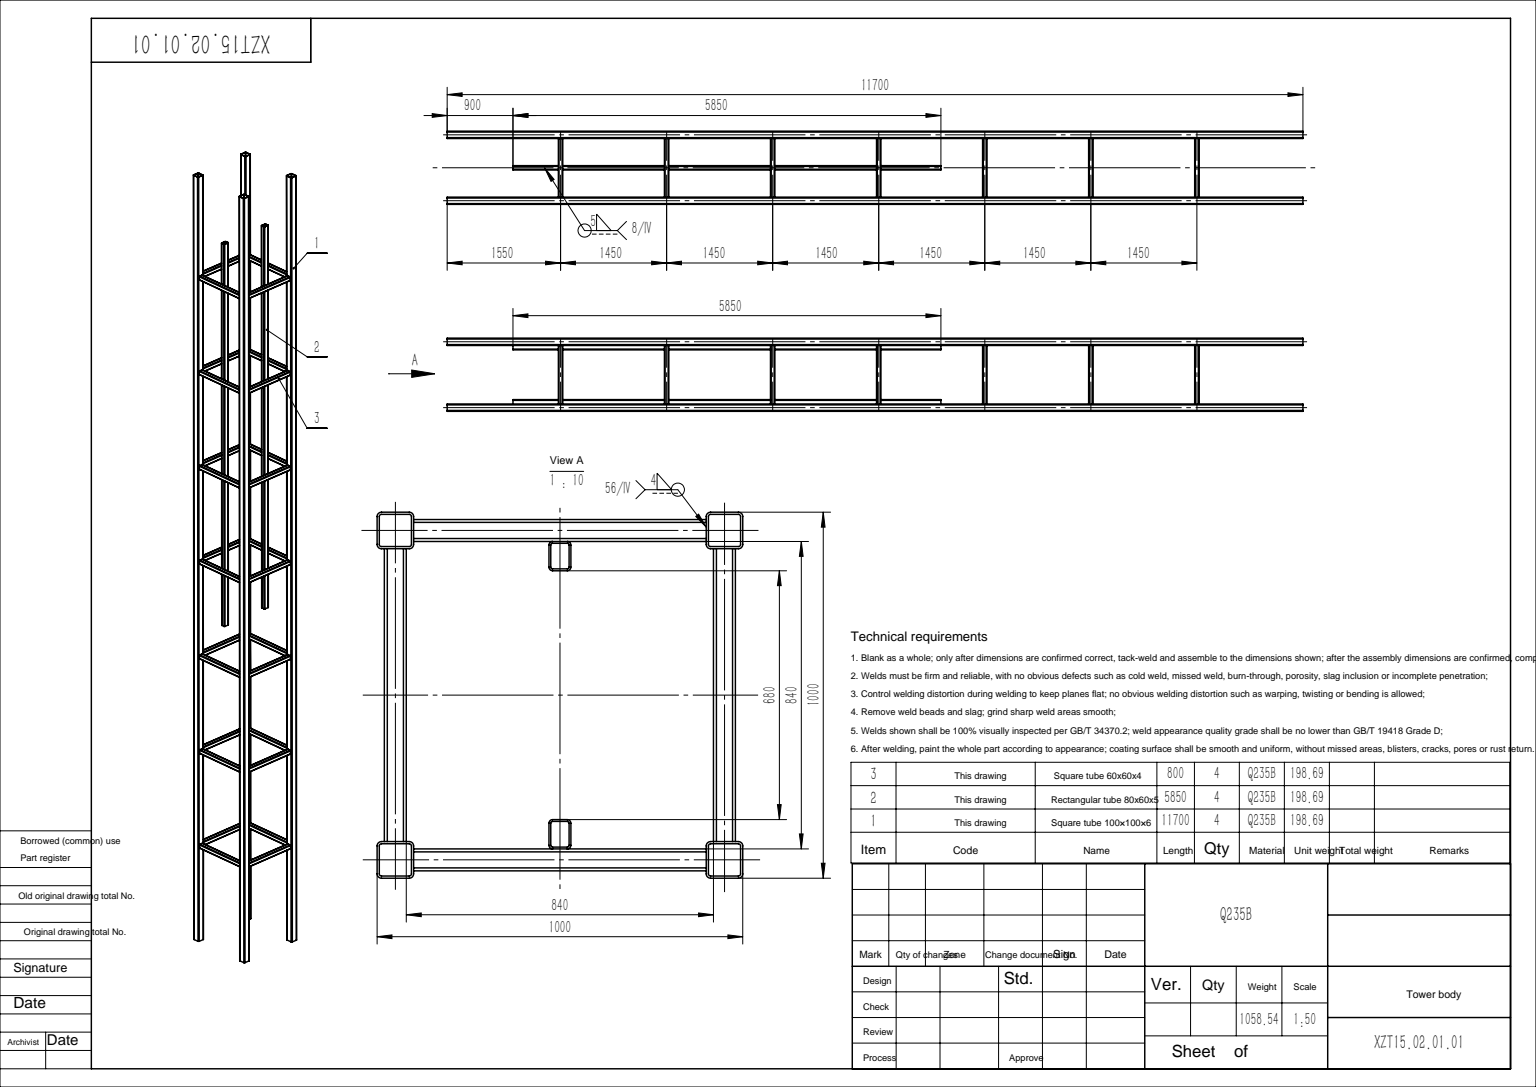
SolidWorks part; units mm, degrees
material "Q235B"
ref_plane "Front Plane" through (0, 0, 0) normal (0, 0, 1) x (1, 0, 0)
ref_plane "Top Plane" through (0, 0, 0) normal (0, 1, 0) x (1, 0, 0)
ref_plane "Right Plane" through (0, 0, 0) normal (1, 0, 0) x (0, 0, -1)
sketch3d "3DSketch1"
  line L0 (450, 0, 0) -> (-450, 0, 0)
  line L1 (0, 0, 450) -> (0, 0, -450)
  line L2 (450, 0, 450) -> (-450, 0, 450)
  line L3 (450, 0, -450) -> (-450, 0, -450)
  line L4 (-450, 0, 450) -> (-450, 0, -450)
  line L5 (450, 0, 450) -> (450, 0, -450)
  line L6 (450, 0, 450) -> (450, 11700, 450)
  line L7 (450, 0, -450) -> (450, 11700, -450)
  line L8 (-450, 0, -450) -> (-450, 11700, -450)
  line L9 (-450, 0, 450) -> (-450, 11700, 450)
  line L10 (-450, 1550, -450) -> (-450, 1550, 450)
  line L11 (-450, 1550, 450) -> (450, 1550, 450)
  line L12 (450, 1550, 450) -> (450, 1550, -450)
  line L13 (450, 1550, -450) -> (-450, 1550, -450)
  line L14 (-380, 0, 0) -> (-380, 900, 0)
  line L15 (380, 0, 0) -> (380, 900, 0)
  line L16 (-380, 900, 0) -> (-380, 6750, 0)
  line L17 (380, 900, 0) -> (380, 6750, 0)
  point P4 (0, 0, 0)
  point P8 (0, 0, 0)
  point P10 (0, 0, 450)
  point P13 (0, 0, -450)
  point P14 (-450, 0, 0)
  point P16 (450, 0, 0)
  dimension "D1" = 900
  dimension "D2" = 11700
  dimension "D3" = 1550
  dimension "D4" = 900
  dimension "D5" = 5850
  dimension "D6" = 70
  dimension "D7" = 70
other "GB/T 6728-2002 square hollow section 100×100×6(1)"
ref_plane "Plane1" through (-450, 0, -450) normal (0, 1, 0) x (1, 0, 0)
sketch "Sketch1" plane through (-450, 0, -450) normal (0, 1, 0) x (1, 0, 0)
  line L0 (-38, -44) -> (38, -44)
  line L1 (-44, -38) -> (-44, 38)
  line L2 (38, 44) -> (-38, 44)
  line L3 (44, 38) -> (44, -38)
  line L4 (-38, -50) -> (38, -50)
  line L5 (-50, -38) -> (-50, 38)
  line L6 (38, 50) -> (-38, 50)
  line L7 (50, 38) -> (50, -38)
  arc A0 (50, 38) -> (38, 50) centre (38, 38) ccw
  arc A1 (38, -50) -> (50, -38) centre (38, -38) ccw
  arc A2 (-50, -38) -> (-38, -50) centre (-38, -38) ccw
  arc A3 (-38, 50) -> (-50, 38) centre (-38, 38) ccw
  arc A4 (-38, 44) -> (-44, 38) centre (-38, 38) ccw
  arc A5 (44, 38) -> (38, 44) centre (38, 38) ccw
  arc A6 (38, -44) -> (44, -38) centre (38, -38) ccw
  arc A7 (-44, -38) -> (-38, -44) centre (-38, -38) ccw
  point P0 (-50, 0)
  point P1 (50, 0)
  point P2 (0, 50)
  point P3 (0, -50)
  point P4 (0, 0)
  point P5 (-50, -50)
  point P6 (50, -50)
  point P7 (50, 50)
  point P8 (-50, 50)
  point P33 (0, 0)
  dimension "D1" = 12
  dimension "Thickness" = 6
  dimension "V_leg" = 100
other "GB/T 6728-2002 square hollow section 60×60×4(1)"
ref_plane "Plane2" through (-450, 1550, -450) normal (0, 0, 1) x (1, 0, 0)
sketch "Sketch12" plane through (-450, 1550, -450) normal (0, 0, 1) x (1, 0, 0)
  line L0 (-22, -26) -> (22, -26)
  line L1 (-26, -22) -> (-26, 22)
  line L2 (22, 26) -> (-22, 26)
  line L3 (26, 22) -> (26, -22)
  line L4 (-22, -30) -> (22, -30)
  line L5 (-30, -22) -> (-30, 22)
  line L6 (22, 30) -> (-22, 30)
  line L7 (30, 22) -> (30, -22)
  arc A0 (30, 22) -> (22, 30) centre (22, 22) ccw
  arc A1 (22, -30) -> (30, -22) centre (22, -22) ccw
  arc A2 (-30, -22) -> (-22, -30) centre (-22, -22) ccw
  arc A3 (-22, 30) -> (-30, 22) centre (-22, 22) ccw
  arc A4 (-22, 26) -> (-26, 22) centre (-22, 22) ccw
  arc A5 (26, 22) -> (22, 26) centre (22, 22) ccw
  arc A6 (22, -26) -> (26, -22) centre (22, -22) ccw
  arc A7 (-26, -22) -> (-22, -26) centre (-22, -22) ccw
  point P0 (-30, 0)
  point P1 (30, 0)
  point P2 (0, 30)
  point P3 (0, -30)
  point P4 (0, 0)
  point P5 (-30, -30)
  point P6 (30, -30)
  point P7 (30, 30)
  point P8 (-30, 30)
  point P33 (0, 0)
  dimension "D1" = 8
  dimension "Thickness" = 4
  dimension "V_leg" = 60
other "GB/T 6728-2002 rectangular hollow section 80X60X5(1)"
ref_plane "Plane3" through (-380, 900, 0) normal (0, 1, 0) x (0, 0, -1)
sketch "Sketch14" plane through (-380, 900, 0) normal (0, 1, 0) x (0, 0, -1)
  line L0 (-20, -35) -> (20, -35)
  line L1 (-25, -30) -> (-25, 30)
  line L2 (20, 35) -> (-20, 35)
  line L3 (25, 30) -> (25, -30)
  line L4 (-20, -40) -> (20, -40)
  line L5 (-30, -30) -> (-30, 30)
  line L6 (20, 40) -> (-20, 40)
  line L7 (30, 30) -> (30, -30)
  arc A0 (30, 30) -> (20, 40) centre (20, 30) ccw
  arc A1 (20, -40) -> (30, -30) centre (20, -30) ccw
  arc A2 (-30, -30) -> (-20, -40) centre (-20, -30) ccw
  arc A3 (-20, 40) -> (-30, 30) centre (-20, 30) ccw
  arc A4 (-20, 35) -> (-25, 30) centre (-20, 30) ccw
  arc A5 (25, 30) -> (20, 35) centre (20, 30) ccw
  arc A6 (20, -35) -> (25, -30) centre (20, -30) ccw
  arc A7 (-25, -30) -> (-20, -35) centre (-20, -30) ccw
  point P0 (0, 40)
  point P1 (30, 0)
  point P2 (0, -40)
  point P3 (-30, 0)
  point P4 (-30, 40)
  point P5 (30, 40)
  point P6 (30, -40)
  point P7 (-30, -40)
  point P8 (0, 0)
  point P33 (0, 0)
  dimension "D1" = 10
  dimension "Thickness" = 5
  dimension "V_leg" = 80
  dimension "H_leg" = 60
other "Trim/Extend1"
pattern_linear "LinearPattern1" count 7 spacing 1450 along (0, 1, 0) of bodies 118 119 117 116
